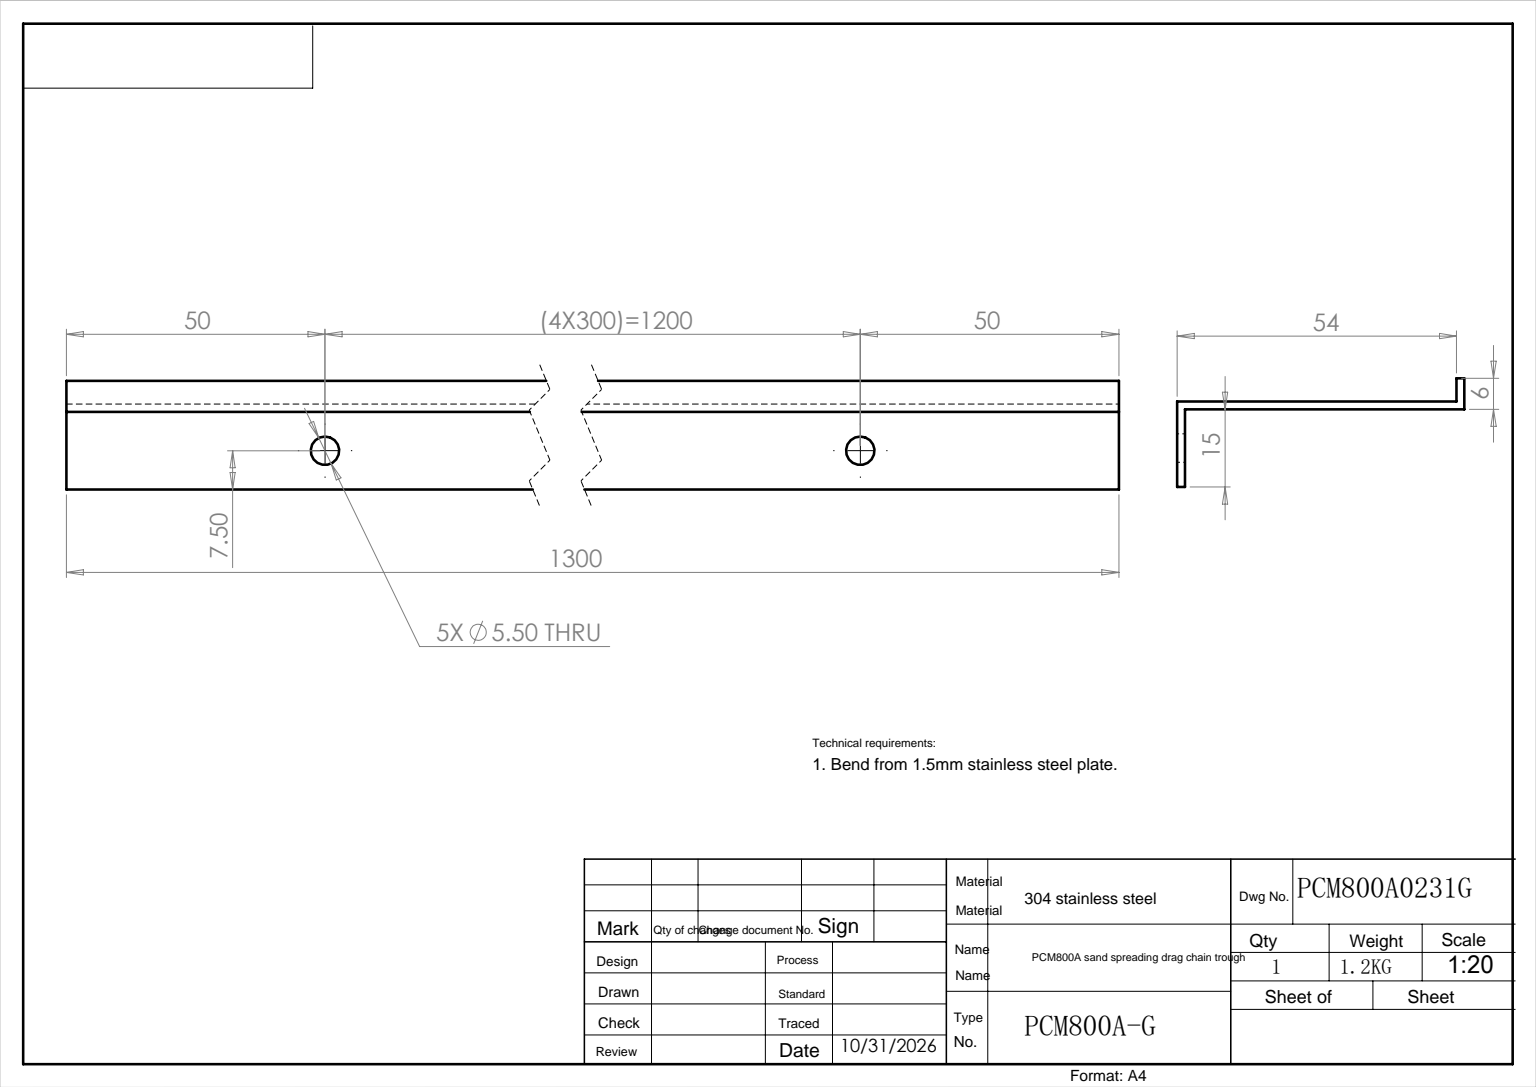
from build123d import *

# Parameters (mm, degrees)
EXTRUDE_1_DEPTH     = 1300
SKETCH_2_R          = 2.75
CUT_EXTRUDE_1_DEPTH = 10


with BuildPart() as part:
    # 草图1 → 拉伸-薄壁1 (new body)
    with BuildSketch(Plane.XY):
        Polygon((54, 6), (54, 0), (0, 0), (0, -15), (-1.5, -15), (-1.5, 1.5), (52.5, 1.5), (52.5, 6), align=None)
    extrude(amount=EXTRUDE_1_DEPTH)

    # 草图2 → 切除-拉伸1 (cut)
    with BuildSketch(Plane(origin=(0, 0, 0), x_dir=(0, 0, -1), z_dir=(1, 0, 0))):
        with Locations(Location((-1250, -7.5, 0), (0, 0, 90))):
            Circle(SKETCH_2_R)
        with Locations(Location((-950, -7.5, 0), (0, 0, 90))):
            Circle(SKETCH_2_R)
        with Locations(Location((-650, -7.5, 0), (0, 0, 90))):
            Circle(SKETCH_2_R)
        with Locations(Location((-350, -7.5, 0), (0, 0, 90))):
            Circle(SKETCH_2_R)
        with Locations(Location((-50, -7.5, 0), (0, 0, 90))):
            Circle(SKETCH_2_R)
    extrude(amount=-CUT_EXTRUDE_1_DEPTH, mode=Mode.SUBTRACT)


solid = part.part
